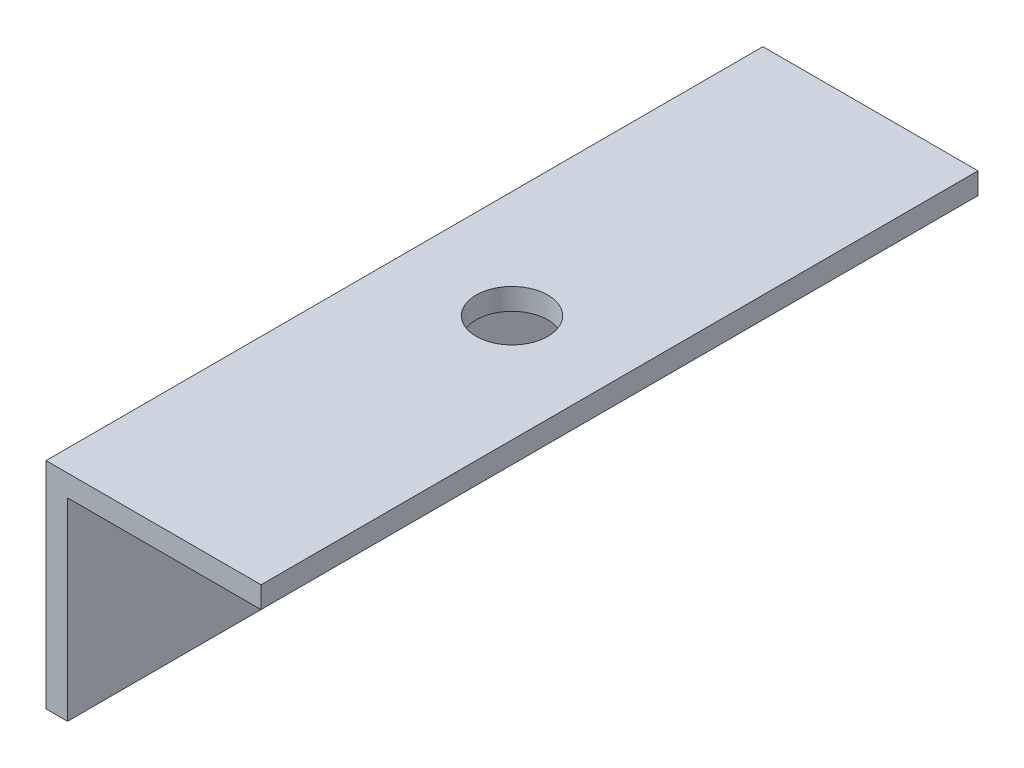
from build123d import *

# Parameters (mm, degrees)
EXTRUDE_1_DEPTH     = 100
CUT_EXTRUDE_1_DEPTH = 10


with BuildPart() as part:
    # 草图1 → 凸台-拉伸1 (new body)
    with BuildSketch(Plane.XY):
        Polygon((0, 0), (30, 0), (30, -3), (3, -3), (3, -30), (0, -30), align=None)
    extrude(amount=EXTRUDE_1_DEPTH)

    # 草图2 → 切除-拉伸1 (cut)
    with BuildSketch(Plane(origin=(0, 0, 0), x_dir=(1, 0, 0), z_dir=(0, 1, 0))):
        with BuildLine():
            ThreePointArc((20, -50), (18.535533906, -46.464466094), (15, -45))
            Line((15, -45), (15, -55))
            ThreePointArc((15, -55), (18.535533906, -53.535533906), (20, -50))
        make_face()
        with BuildLine():
            Line((15, -55), (15, -45))
            ThreePointArc((15, -45), (10, -50), (15, -55))
        make_face()
    extrude(amount=-CUT_EXTRUDE_1_DEPTH, mode=Mode.SUBTRACT)


solid = part.part
